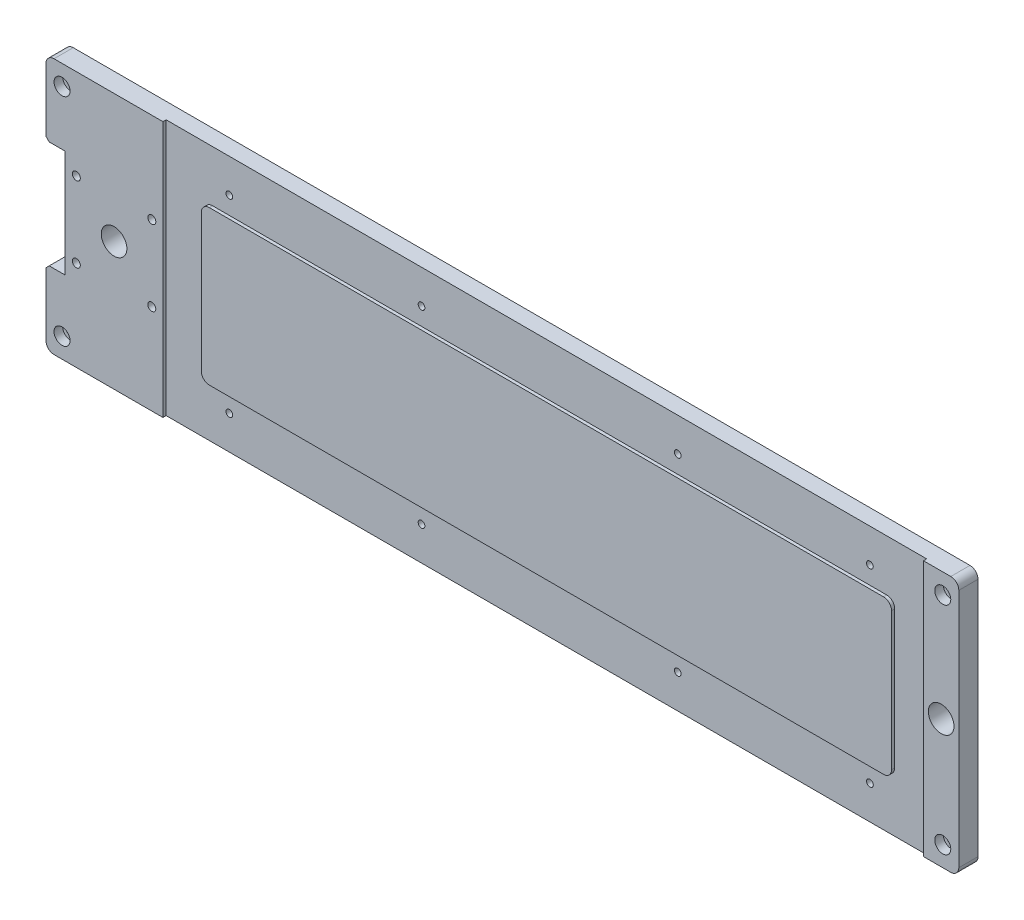
from build123d import *

# Parameters (mm, degrees)
SKETCH1_W                                           = 570
SKETCH1_H                                           = 160
BOSS_EXTRUDE1_DEPTH                                 = 12
SKETCH2_W                                           = 24
SKETCH2_H                                           = 246.506816481
SKETCH2_W_2                                         = 20
SKETCH2_H_2                                         = 260.473208351
CUT_EXTRUDE1_DEPTH                                  = 2
SKETCH3_W                                           = 431
SKETCH3_H                                           = 32
CUT_EXTRUDE2_DEPTH                                  = 2
SKETCH4_W                                           = 12
SKETCH4_H                                           = 67
CUT_EXTRUDE3_DEPTH                                  = 297.258333216
M5_TAPPED_HOLE1_D                                   = 4.2
FILLET1_R                                           = 5
FILLET2_R                                           = 5
CHAMFER1_SIZE                                       = 2
CBORE_FOR_M5_HEX_SOCKET_HEAD_CAP_SCREW1_D           = 5.5
CBORE_FOR_M5_HEX_SOCKET_HEAD_CAP_SCREW1_CBORE_D     = 10
CBORE_FOR_M5_HEX_SOCKET_HEAD_CAP_SCREW1_CBORE_DEPTH = 5.4
SKETCH13_R                                          = 8
CUT_EXTRUDE4_DEPTH                                  = 18
SKETCH14_R                                          = 2.5
CUT_EXTRUDE5_DEPTH                                  = 12
SKETCH15_R                                          = 8
CUT_EXTRUDE6_DEPTH                                  = 12


with BuildPart() as part:
    # Sketch1 → Boss-Extrude1 (new body)
    with BuildSketch(Plane.XY):
        Rectangle(SKETCH1_W, SKETCH1_H)
    extrude(amount=BOSS_EXTRUDE1_DEPTH)

    # Sketch2 → Cut-Extrude1 (cut)
    with BuildSketch(Plane.XY.offset(12)):
        with Locations((-200, -10.474793902)):
            Rectangle(SKETCH2_W, SKETCH2_H)
        with Locations((253, -9.078154715)):
            Rectangle(SKETCH2_W_2, SKETCH2_H_2)
    extrude(amount=-CUT_EXTRUDE1_DEPTH, mode=Mode.SUBTRACT)

    # Sketch3 → Cut-Extrude2 (cut)
    with BuildSketch(Plane.XY.offset(12)):
        with Locations((27.5, 64)):
            Rectangle(SKETCH3_W, SKETCH3_H)
        with Locations((27.5, -64)):
            Rectangle(SKETCH3_W, SKETCH3_H)
    extrude(amount=-CUT_EXTRUDE2_DEPTH, mode=Mode.SUBTRACT)

    # Sketch4 → Cut-Extrude3 (cut, through all)
    with BuildSketch(Plane.XY.offset(12)):
        with Locations((-279, 0)):
            Rectangle(SKETCH4_W, SKETCH4_H)
    extrude(amount=-CUT_EXTRUDE3_DEPTH, mode=Mode.SUBTRACT)

    # M5 Tapped Hole1 (through all)
    with Locations(Plane.XY.offset(10)):
        with Locations((227.5, -59), (107.5, -59), (-172.5, -59), (-52.5, -59), (-172.5, 59), (-52.5, 59), (107.5, 59), (227.5, 59)):
            Hole(M5_TAPPED_HOLE1_D / 2)

    # Fillet1
    fillet1_edges = [part.edges().sort_by_distance(p)[0] for p in [
        (-188, 48, 11),
        (243, 48, 11),
        (-188, -48, 11),
        (243, -48, 11),
    ]]
    fillet(fillet1_edges, radius=FILLET1_R)

    # Fillet2
    fillet2_edges = [part.edges().sort_by_distance(p)[0] for p in [
        (285, -80, 6),
        (-285, -80, 6),
        (-285, 80, 6),
        (285, 80, 6),
    ]]
    fillet(fillet2_edges, radius=FILLET2_R)

    # Chamfer1
    chamfer1_edges = [part.edges().sort_by_distance(p)[0] for p in [
        (-285, -33.5, 6),
        (-285, 33.5, 6),
    ]]
    chamfer(chamfer1_edges, length=CHAMFER1_SIZE)

    # CBORE for M5 Hex Socket Head Cap Screw1 (through all)
    with Locations(Plane.XY.offset(12)):
        with Locations((275, 67.5), (-275, -67.5), (-275, 67.5), (275, -67.5)):
            CounterBoreHole(CBORE_FOR_M5_HEX_SOCKET_HEAD_CAP_SCREW1_D / 2, CBORE_FOR_M5_HEX_SOCKET_HEAD_CAP_SCREW1_CBORE_D / 2, CBORE_FOR_M5_HEX_SOCKET_HEAD_CAP_SCREW1_CBORE_DEPTH)

    # Sketch13 → Cut-Extrude4 (cut)
    with BuildSketch(Plane.XY.offset(12)):
        with Locations((-242.5, 0)):
            Circle(SKETCH13_R)
    extrude(amount=-CUT_EXTRUDE4_DEPTH, mode=Mode.SUBTRACT)

    # Sketch14 → Cut-Extrude5 (cut)
    with BuildSketch(Plane(origin=(0, 0, 0), x_dir=(-1, 0, 0), z_dir=(0, 0, -1))):
        with Locations((218.93, -23.570000001)):
            Circle(SKETCH14_R)
        with Locations((266.07, -23.569995906)):
            Circle(SKETCH14_R)
        with Locations((266.069995906, 23.570004094)):
            Circle(SKETCH14_R)
        with Locations((218.929995906, 23.569999999)):
            Circle(SKETCH14_R)
    extrude(amount=-CUT_EXTRUDE5_DEPTH, mode=Mode.SUBTRACT)

    # Sketch15 → Cut-Extrude6 (cut)
    with BuildSketch(Plane.XY.offset(12)):
        with Locations((274, 0)):
            Circle(SKETCH15_R)
    extrude(amount=-CUT_EXTRUDE6_DEPTH, mode=Mode.SUBTRACT)


solid = part.part
